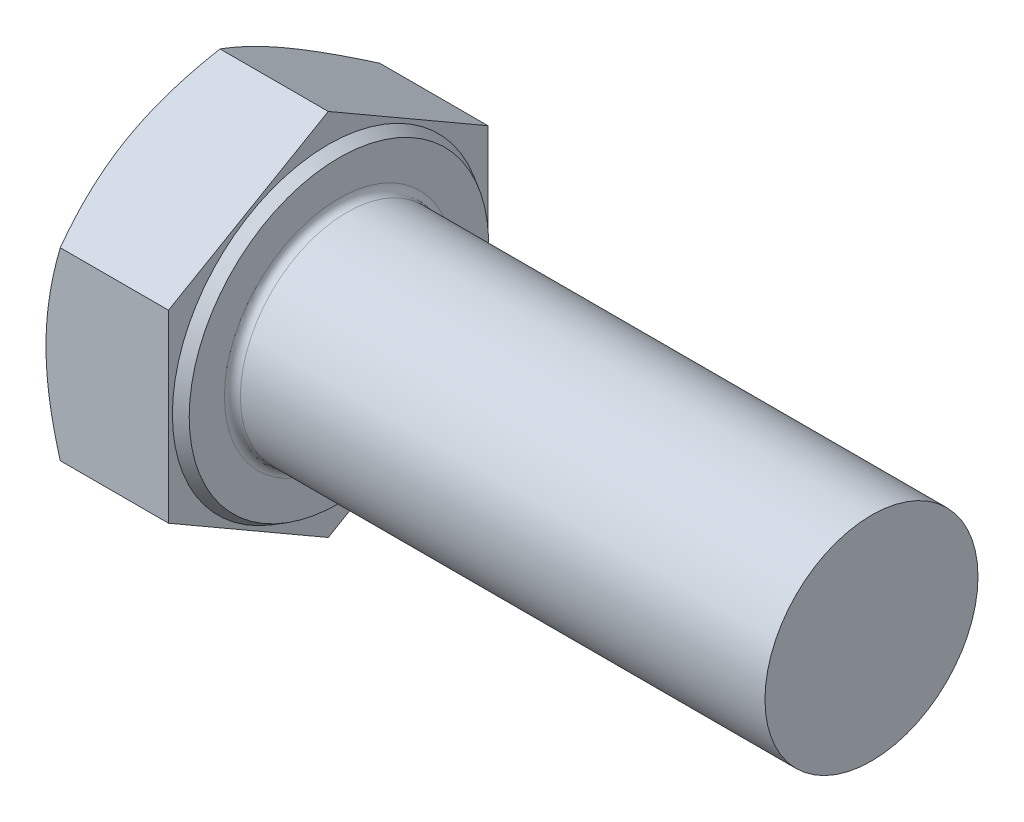
SolidWorks part; units mm, degrees
ref_plane "前视" through (0, 0, 0) normal (0, 0, 1) x (1, 0, 0)
ref_plane "上视" through (0, 0, 0) normal (0, 1, 0) x (1, 0, 0)
ref_plane "右视" through (0, 0, 0) normal (1, 0, 0) x (0, 0, -1)
sketch "草图1" plane through (0, 0, 0) normal (1, 0, 0) x (0, 0, -1)
  line L0 (12, 6.9282) -> (12, -6.9282)
  line L1 (-12, 6.9282) -> (-12, -6.9282)
  line L2 (12, -6.9282) -> (0, -13.8564)
  line L3 (0, -13.8564) -> (-12, -6.9282)
  line L4 (12, 6.9282) -> (0, 13.8564)
  line L5 (0, 13.8564) -> (-12, 6.9282)
  circle A0 centre (0, 0) radius 13.375 construction
  dimension "e" = 26.75
  dimension "s" = 24
  dimension "D2" = 120
  dimension "D3" = 12
  dimension "D4" = 12
  dimension "D5" = 12
extrude "基体-拉伸" add sketch "草图1" along normal blind 10
sketch "草图2" plane through (0, 0, 0) normal (0, 0, 1) x (1, 0, 0)
  line L0 (0, 6.9282) -> (0, -6.9282) construction
  line L1 (0, 0) -> (50, 0)
  line L2 (0, 0) -> (0, 8)
  line L3 (0, 8) -> (12, 8)
  line L4 (50, 0) -> (50, 6.268)
  line L5 (10, 13.8564) -> (10, 6.9282) construction
  line L7 (0, 0) -> (66, 0) construction
  line L8 (50, -6.268) -> (12, -8) construction
  line L9 (0, -8) -> (12, -8) construction
  line L10 (12, 8) -> (12, 0) construction
  line L11 (12, 15.24) -> (12, -1.27) construction
  line L12 (10, 6.9282) -> (10, -6.9282) construction
  line L13 (12, 8) -> (50, 8)
  line L14 (50, 8) -> (50, 6.268)
  dimension "l" = 40
  dimension "d" = 16
  dimension "Minor_dia" = 12.536
  dimension "p" = 2
  dimension "b" = 38
  dimension "ds" = 16
revolve "凸台-旋转1" add sketch "草图2" angle 360 about L7
cosmetic thread "螺旋线1" parameters "Thread_length"=38, "Thread_minor"=12.536
sketch "草图3" plane through (0, 0, 0) normal (0, 0, 1) x (1, 0, 0)
  line L0 (0, 12) -> (3.9585, 18.8564)
  line L1 (0, 13.8564) -> (0, 6.9282) construction
  line L2 (3.9585, 18.8564) -> (3.9585, 23.8564)
  line L3 (3.9585, 23.8564) -> (-10, 23.8564)
  line L4 (-10, 23.8564) -> (-10, 12)
  line L5 (-10, 12) -> (0, 12)
  line L6 (0, 0) -> (99.06, 0) construction
  line L7 (10, 13.8564) -> (0, 13.8564) construction
  dimension "D1" = 12
  dimension "D2" = 5
  dimension "D3" = 10
  dimension "D4" = 5
  dimension "Head_ch_ang" = 30
revolve "切除-旋转1" cut sketch "草图3" angle 360 about L6
sketch "草图4" plane through (0, 0, 0) normal (0, 0, 1) x (1, 0, 0)
  line L0 (10, 0) -> (10, 11.245) construction
  line L2 (10, -8) -> (10, 8) construction
  line L3 (10, 13.8564) -> (10, 6.9282) construction
  line L4 (10, 11.245) -> (9.2, 11.7069)
  line L5 (0, 0) -> (95.25, 0) construction
  line L6 (0, 0) -> (66, 0) construction
  line L9 (9.2, 11.7069) -> (9.2, 13.8564)
  line L10 (10, 13.8564) -> (1.0718, 13.8564) construction
  line L11 (9.2, 13.8564) -> (10, 13.8564)
  line L12 (10, 13.8564) -> (10, 11.245)
  dimension "D1" = 120
  dimension "c" = 0.8
  dimension "dw" = 22.49
revolve "切除-旋转3" cut sketch "草图4" angle 360 about L5
fillet "圆角" radius 0.6 1 edges at (10, 0, -8)
sketch "草图6" plane through (0, 0, 0) normal (0, 0, 1) x (1, 0, 0)
  line L0 (0, 0) -> (50, 0) construction
  line L1 (50, -8) -> (50, 8) construction
  line L2 (50, 0) -> (50, 8) construction
  line L4 (49, 8) -> (51, 8)
  line L5 (49, 8) -> (50, 6.2679)
  line L6 (50, 6.2679) -> (51, 8)
  dimension "D1" = 2
revolve "切除-旋转4" [suppressed] cut sketch "草图6" angle 360 about L0
pattern_linear "阵列(线性)1" [suppressed]
